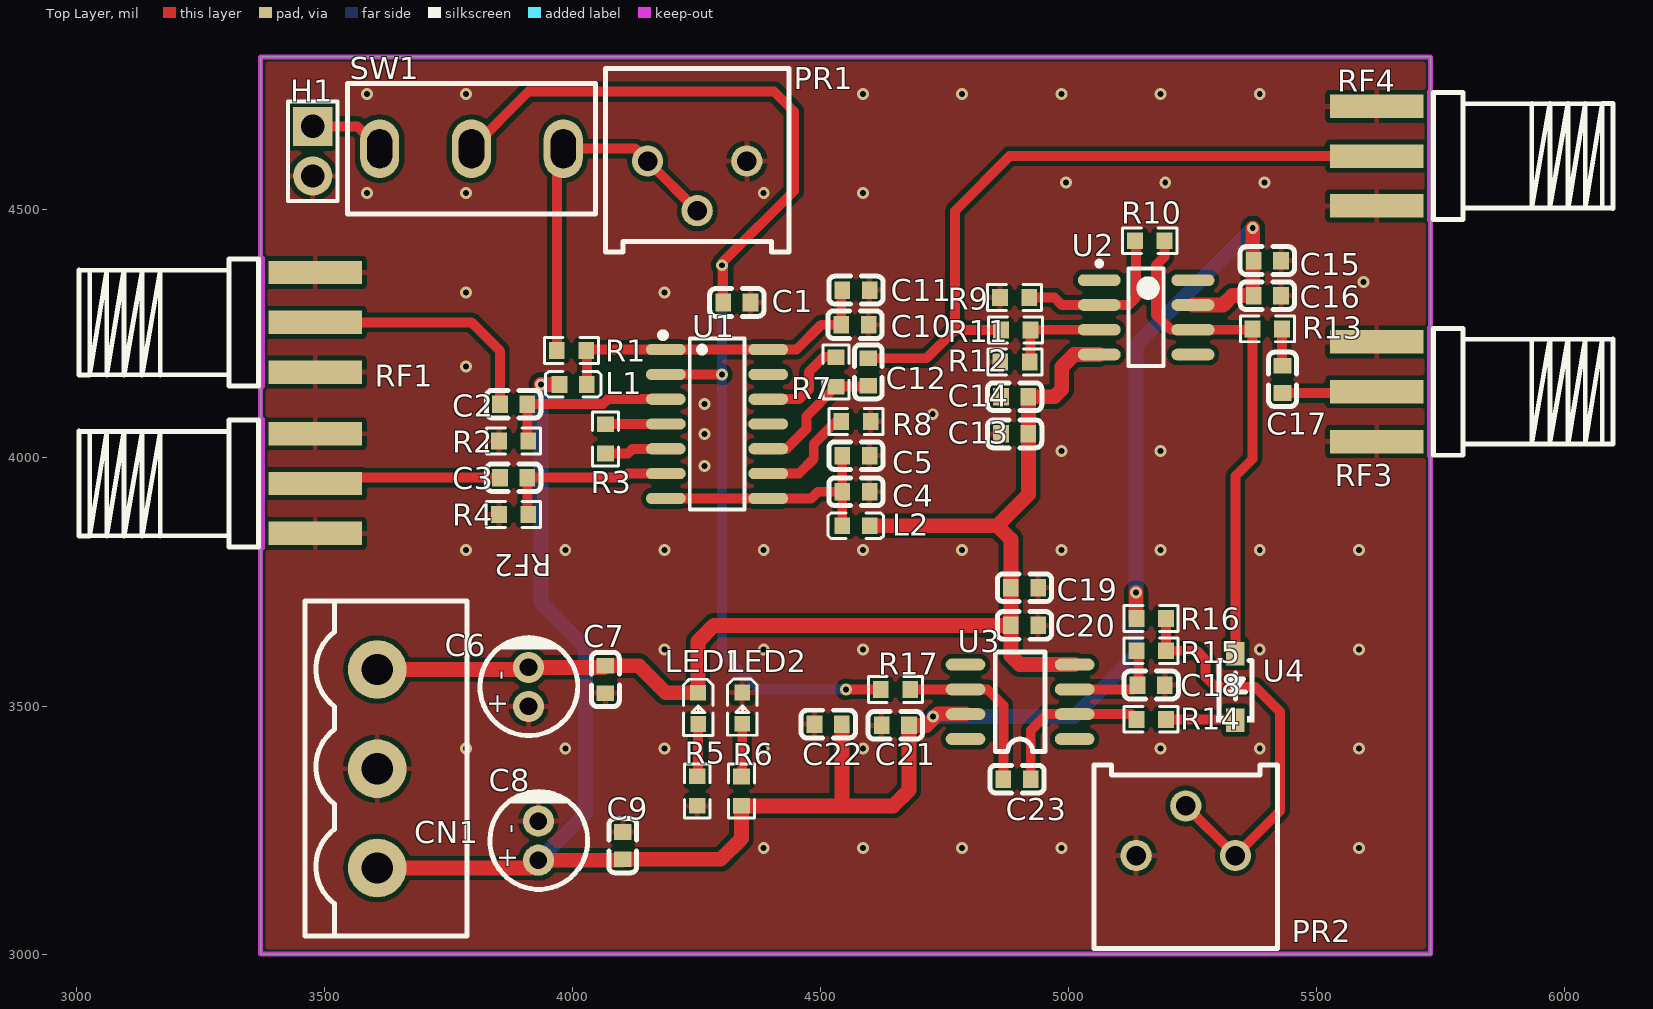
[diagram p0: Top Layer view]
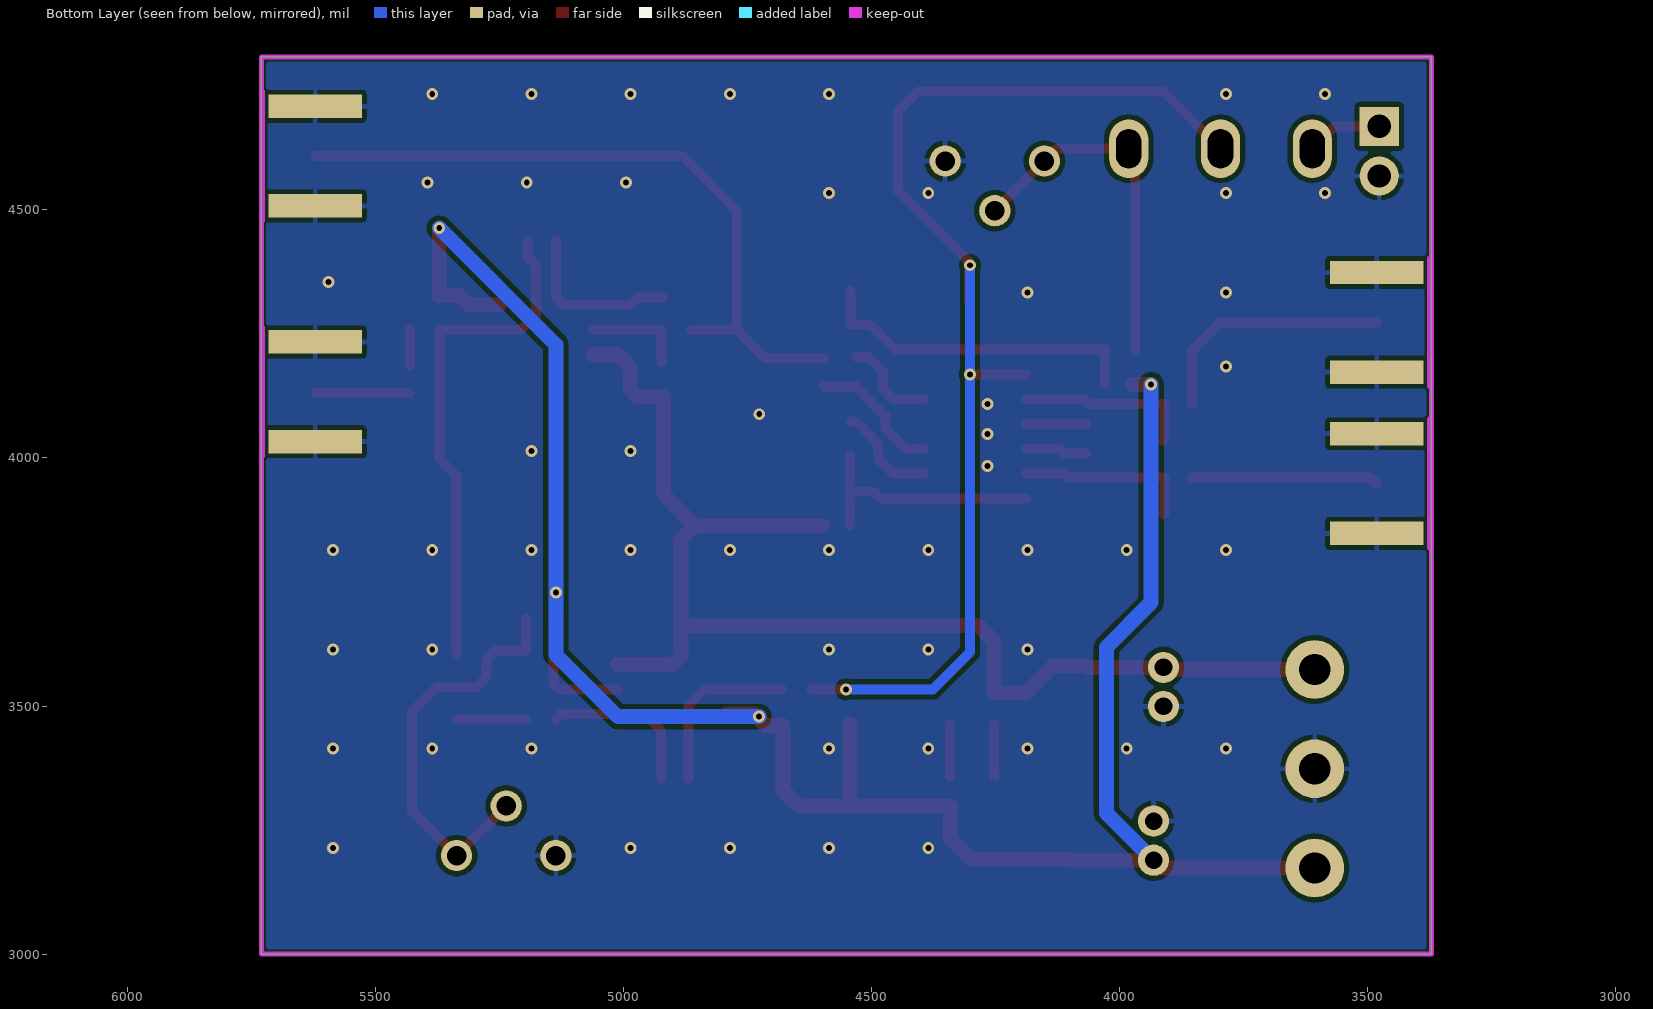
[diagram p1: Bottom Layer view, seen from below]
# Altium PCB MISC52012.pcbdoc
Units mil, origin at the board's own origin, x right, y up, seen from the top; angles counter-clockwise.
Board outline 2358.5 x 1808.5 mil, 2 copper layers (Top Layer, Bottom Layer), stack 62.206 mil thick; 57 components, 30 nets, 154 pads, 59 vias.

## Layer stack, top to bottom
Top Solder Mask Layer: solder mask 0.394, Dk 3.3
Top Layer: signal copper 1.379
Dielectric 1: surface 59.449, FR4, Dk 4.5
Bottom Layer: signal copper 1.378
Bottom Solder Mask Layer: solder mask 0.394, Dk 3.3

## Board outline
3371.1,4808.5 3371.1,3000 5729.61,3000 5729.61,4808.5

## Design rules (kind name [scope] priority, off if disabled: settings)
BoardOutlineClearance copperThickness2oz_1 [All] p2 off: genericclearance=7.99 ignorepadtopadclearanceinfootprint=FALSE except(0: Arc-SplitContinuation Track-SplitContinuation SMDPad-SplitContinuation THPad-SplitContinuation Via-SplitContinuation Fill-SplitContinuation Region-SplitContinuation Poly-SplitContinuation Text-SplitContinuation Hole-SplitContinuation; 5.98: Arc-CutoutEdge Track-CutoutEdge SMDPad-CutoutEdge THPad-CutoutEdge Via-CutoutEdge Text-CutoutEdge; 6.9: Hole-OutlineEdge Hole-CutoutEdge; 10: Poly-OutlineEdge Poly-CutoutEdge; 11.81: Arc-OutlineEdge Track-OutlineEdge SMDPad-OutlineEdge THPad-OutlineEdge Via-OutlineEdge Fill-OutlineEdge Region-OutlineEdge Text-OutlineEdge Fill-CutoutEdge Region-CutoutEdge)
BoardOutlineClearance Plane_innerPlane_1 [All] p4 off: genericclearance=4.02 ignorepadtopadclearanceinfootprint=FALSE except(0: Arc-SplitContinuation Track-SplitContinuation SMDPad-SplitContinuation THPad-SplitContinuation Via-SplitContinuation Fill-SplitContinuation Region-SplitContinuation Poly-SplitContinuation Text-SplitContinuation Hole-SplitContinuation; 5.98: Arc-CutoutEdge Track-CutoutEdge SMDPad-CutoutEdge THPad-CutoutEdge Via-CutoutEdge Text-CutoutEdge; 6.9: Hole-OutlineEdge Hole-CutoutEdge; 10: Poly-OutlineEdge Poly-CutoutEdge; 11.81: Arc-OutlineEdge Track-OutlineEdge SMDPad-OutlineEdge THPad-OutlineEdge Via-OutlineEdge Fill-OutlineEdge Region-OutlineEdge Text-OutlineEdge Fill-CutoutEdge Region-CutoutEdge)
BoardOutlineClearance Copper_copperRegion_1 [All] p6 off: genericclearance=4.02 ignorepadtopadclearanceinfootprint=FALSE except(0: Arc-SplitContinuation Track-SplitContinuation SMDPad-SplitContinuation THPad-SplitContinuation Via-SplitContinuation Fill-SplitContinuation Region-SplitContinuation Poly-SplitContinuation Text-SplitContinuation Hole-SplitContinuation; 5.98: Arc-CutoutEdge Track-CutoutEdge SMDPad-CutoutEdge THPad-CutoutEdge Via-CutoutEdge Text-CutoutEdge; 6.9: Hole-OutlineEdge Hole-CutoutEdge; 10: Poly-OutlineEdge Poly-CutoutEdge; 11.81: Arc-OutlineEdge Track-OutlineEdge SMDPad-OutlineEdge THPad-OutlineEdge Via-OutlineEdge Fill-OutlineEdge Region-OutlineEdge Text-OutlineEdge Fill-CutoutEdge Region-CutoutEdge)
BoardOutlineClearance copperThickness1oz_1 [All] p8: genericclearance=4.02 ignorepadtopadclearanceinfootprint=FALSE except(0: Arc-SplitContinuation Track-SplitContinuation SMDPad-SplitContinuation THPad-SplitContinuation Via-SplitContinuation Fill-SplitContinuation Region-SplitContinuation Poly-SplitContinuation Text-SplitContinuation Hole-SplitContinuation; 5.98: Arc-CutoutEdge Track-CutoutEdge SMDPad-CutoutEdge THPad-CutoutEdge Via-CutoutEdge Text-CutoutEdge; 6.9: Hole-OutlineEdge Hole-CutoutEdge; 10: Poly-OutlineEdge Poly-CutoutEdge; 11.81: Arc-OutlineEdge Track-OutlineEdge SMDPad-OutlineEdge THPad-OutlineEdge Via-OutlineEdge Fill-OutlineEdge Region-OutlineEdge Text-OutlineEdge Fill-CutoutEdge Region-CutoutEdge)
Clearance copperThickness2oz [All] p1 off: gap=7.99 ignorepadtopadclearanceinfootprint=FALSE except(5.98: SMDPad-Track SMDPad-SMDPad THPad-Track SMDPad-THPad THPad-THPad Track-Via SMDPad-Via THPad-Via Via-Via Fill-SMDPad Region-SMDPad Fill-THPad Region-THPad Fill-Via Region-Via Fill-Fill Fill-Region Region-Region Arc-Track Arc-SMDPad Arc-THPad Arc-Via Fill-Arc Region-Arc Arc-Arc Text-Track SMDPad-Text Text-THPad Text-Via Fill-Text Region-Text Arc-Text Text-Text; 6.9: Hole-Track Hole-SMDPad Hole-THPad Hole-Via Fill-Hole Region-Hole Hole-Arc Hole-Text; 10: Poly-Track Poly-SMDPad Poly-THPad Poly-Via Poly-Fill Poly-Region Poly-Poly Poly-Arc Poly-Text Poly-Hole; 11.81: Fill-Track Region-Track)
Clearance Plane_innerPlane [All] p3 off: gap=4.02 ignorepadtopadclearanceinfootprint=FALSE except(5.98: SMDPad-Track SMDPad-SMDPad THPad-Track SMDPad-THPad THPad-THPad Track-Via SMDPad-Via THPad-Via Via-Via Fill-SMDPad Region-SMDPad Fill-THPad Region-THPad Fill-Via Region-Via Fill-Fill Fill-Region Region-Region Arc-Track Arc-SMDPad Arc-THPad Arc-Via Fill-Arc Region-Arc Arc-Arc Text-Track SMDPad-Text Text-THPad Text-Via Fill-Text Region-Text Arc-Text Text-Text; 6.9: Hole-Track Hole-SMDPad Hole-THPad Hole-Via Fill-Hole Region-Hole Hole-Arc Hole-Text; 10: Poly-Track Poly-SMDPad Poly-THPad Poly-Via Poly-Fill Poly-Region Poly-Poly Poly-Arc Poly-Text Poly-Hole; 11.81: Fill-Track Region-Track)
Clearance Copper_copperRegion [All] p5 off: gap=4.02 ignorepadtopadclearanceinfootprint=FALSE except(5.98: SMDPad-Track SMDPad-SMDPad THPad-Track SMDPad-THPad THPad-THPad Track-Via SMDPad-Via THPad-Via Via-Via Fill-SMDPad Region-SMDPad Fill-THPad Region-THPad Fill-Via Region-Via Fill-Fill Fill-Region Region-Region Arc-Track Arc-SMDPad Arc-THPad Arc-Via Fill-Arc Region-Arc Arc-Arc Text-Track SMDPad-Text Text-THPad Text-Via Fill-Text Region-Text Arc-Text Text-Text; 6.9: Hole-Track Hole-SMDPad Hole-THPad Hole-Via Fill-Hole Region-Hole Hole-Arc Hole-Text; 10: Poly-Track Poly-SMDPad Poly-THPad Poly-Via Poly-Fill Poly-Region Poly-Poly Poly-Arc Poly-Text Poly-Hole; 11.81: Fill-Track Region-Track)
Clearance copperThickness1oz [All] p7: gap=4.02 ignorepadtopadclearanceinfootprint=FALSE except(5.98: SMDPad-Track SMDPad-SMDPad THPad-Track SMDPad-THPad THPad-THPad Track-Via SMDPad-Via THPad-Via Via-Via Fill-SMDPad Region-SMDPad Fill-THPad Region-THPad Fill-Via Region-Via Fill-Fill Fill-Region Region-Region Arc-Track Arc-SMDPad Arc-THPad Arc-Via Fill-Arc Region-Arc Arc-Arc Text-Track SMDPad-Text Text-THPad Text-Via Fill-Text Region-Text Arc-Text Text-Text; 6.9: Hole-Track Hole-SMDPad Hole-THPad Hole-Via Fill-Hole Region-Hole Hole-Arc Hole-Text; 10: Poly-Track Poly-SMDPad Poly-THPad Poly-Via Poly-Fill Poly-Region Poly-Poly Poly-Arc Poly-Text Poly-Hole; 11.81: Fill-Track Region-Track)
DiffPairsRouting differentialPair [All] p1: maxlimit=6 minlimit=6 mostfreqgap=6 toplayer_minwidth=5 toplayer_prefwidth=10 toplayer_maxwidth=100 toplayer_mingap=6 toplayer_prefgap=6 toplayer_maxgap=6 bottomlayer_minwidth=5 bottomlayer_prefwidth=10 bottomlayer_maxwidth=100 bottomlayer_mingap=6 bottomlayer_prefgap=6 bottomlayer_maxgap=6 maxuncoupledlength=10
HoleToHoleClearance otherClearance [All] p1: gap=11.81 allowstackedmicrovias=TRUE
Length netLength [All] p1: minlimit=0 maxlimit=0
PasteMaskExpansion pasteMaskExpansion [All] p1: expansion=0
PlaneConnect innerPlane [All] p1: planeconnectstyle=Relief reliefexpansion=20 reliefentries=4 reliefconductorwidth=10 reliefairgap=10
PolygonConnect copperRegion [All] p1: connectstyle=Relief reliefconductorwidth=10 reliefentries=4 polygonreliefangle="90 Angle" airgapwidth=10 via.connectstyle=Relief via.reliefconductorwidth=10 via.reliefentries=4 via.polygonreliefangle="90 Angle" via.airgapwidth=10
RoutingVias viaSize [All] p1: holewidth=12.01 width=24.02 viastyle="Through Hole" minholewidth=11.81 minwidth=19.68 maxholewidth=248.03 maxwidth=393.7
SolderMaskExpansion solderMaskExpansion [IsVia] p1: expansion=-1000 istentingtop=TRUE
SolderMaskExpansion solderMaskExpansion [All] p2: expansion=2 istentingtop=FALSE
Width copperThickness2oz_2 [All] p1 off: maxlimit=100 minlimit=8 preferedwidth=10
Width copperThickness1oz_2 [All] p2: maxlimit=100 minlimit=5 preferedwidth=10

## Components (designator, comment, footprint, x,y, rotation, side; value= is the part's Value field where it differs from the comment)
C1 "100nF" C0603 4331.1,4313.5 r180 top
C2 "100nF" C0603 3881.1,4108.5 r0 top
C3 "100nF" C0603 3881.1,3960.24 r0 top
C4 "100nF" C0603 4571.1,3931.94 r0 top
C5 "1uF" C0603 4571.1,4004.7 r180 top
C6 "10uF" CAP-TH_BD5.0-P2.00-D0.5-FD-A 3911.1,3538.5 r90 top
C7 "100nF" C0603 4066.1,3553.5 r90 top
C8 "10uF" CAP-TH_BD5.0-P2.00-D0.5-FD-A 3931.1,3228.5 r90 top
C9 "100nF" C0603 4101.1,3218.5 r270 top
C10 "1uF" C0603 4569.1,4268.56 r0 top
C11 "100nF" C0603 4571.1,4338.5 r0 top
C12 "100nF" C0603 4596.1,4173.5 r90 top
C13 "100nF" C0603 4891.1,4048.5 r0 top
C14 "1uF" C0603 4891.1,4123.5 r0 top
C15 "1uF" C0603 5400.45,4397.98 r0 top
C16 "100nF" C0603 5400.45,4327.19 r0 top
C17 "100nF" C0603 5431.1,4158.5 r270 top
C18 "100nF" C0603 5166.33,3542.25 r180 top
C19 "100nF" C0603 4910.99,3738.51 r180 top
C20 "1uF" C0603 4911,3662.53 r180 top
C21 "100nF" C0603 4650.47,3461.07 r180 top
C22 "1uF" C0603 4515.28,3463.51 r180 top
C23 "100nF" C0603 4896,3352.53 r180 top
CN1 "WJ2EDGVC-5.08-03P-14-00A" CONN-TH_3P-P5.08-WJ2EDGVC-3P 3606.1,3373.5 r270 top
H1 "PZ254V-11-02P" HDR-TH_2P-P2.54-V-M 3476.1,4618.5 r270 top
L1 "10uH" L0603 4001.1,4148.5 r0 top
L2 "10uH" L0603 4571.1,3863.5 r180 top
LED1 "" LED_0603 4253.2,3493.3 r270 top
LED2 "" LED_0603 4342.17,3493.79 r270 top
PR1 "10K" R_3386P 4251.1,4598.5 r90 top
PR2 "10K" R_3386P 5236.1,3198.5 r270 top
R1 "10K" R0603 3997.75,4216.58 r180 top
R2 "51R" R0603 3881.11,4034.38 r180 top
R3 "10" R0603 4066.1,4038.5 r90 top
R4 "50R" R0603 3881.11,3886.12 r0 top
R5 "1K" R0603 4251.1,3328.5 r90 top
R6 "1K" R0603 4340.27,3328.37 r90 top
R7 "1K" R0603 4531.1,4173.5 r270 top
R8 "0" R0603 4571.1,4073.5 r180 top
R9 "51R" R0603 4891.1,4323.5 r0 top
R10 "1K" R0603 5163.52,4437.98 r0 top
R11 "10R" R0603 4893.16,4257.98 r0 top
R12 "51R" R0603 4891.78,4193.5 r0 top
R13 "10R" R0603 5400.46,4260.34 r0 top
R14 "1K" R0603 5166.33,3473.17 r0 top
R15 "100" R0603 5166.33,3611.33 r0 top
R16 "3K" R0603 5166.33,3676.47 r180 top
R17 "100" R0603 4650.74,3533.17 r0 top
RF1 "6GHz" SMA-SMD_BWSMA-KE-P001 3481.1,4273.5 r180 top
RF2 "6GHz" SMA-SMD_BWSMA-KE-P001 3481.1,3948.5 r180 top
RF3 "6GHz" SMA-SMD_BWSMA-KE-P001 5621.1,4133.5 r0 top
RF4 "6GHz" SMA-SMD_BWSMA-KE-P001 5621.1,4608.5 r0 top
SW1 "SS-12D10L5" SW-TH_SS-12D10L5 3796.1,4623.5 r180 top
U1 "VCA821ID" SOIC-14_L8.7-W3.9-P1.27-LS6.0-BL 4291.1,4068.5 r270 top
U2 "OPA695" SOIC-8 5156.1,4283.5 r0 top
U3 "OPA820" SOP8 5011,3432.53 r180 top
U4 "1N4150" SOD-123_L2.7-W1.6-LS3.7-RD-1 5336.1,3538.5 r90 top

## Footprints (in the part's own frame and the unit in brackets; to place one, negate y for a bottom-side part, rotate by r counter-clockwise, add the part's x,y. Pads: shape width x height; smd on the part's side, far side on the other; paste and mask are expansions set on the pad)
C0603 [mm]
  rect 0.8x0.9 smd: 1(-0.7,0) 2(0.7,0)
  silkscreen extent -1.39,-0.71 1.39,0.71
CAP-TH_BD5.0-P2.00-D0.5-FD-A [mm]
  round 1.6 hole 0.9 paste+0 mask+0.05: 1(-1,0) 2(1,0)
  silkscreen extent -2.49,-2.52 2.6,2.49
CONN-TH_3P-P5.08-WJ2EDGVC-3P [mm]
  round 3 hole 1.6 paste+0 mask+0.05: 1(-5.08,0) 2(0,0) 3(5.08,0)
  silkscreen extent -8.58,-3.7 8.57,4.6
HDR-TH_2P-P2.54-V-M [mm]
  rect 2x2 hole 1.2: 1(-1.27,0)
  round 2 hole 1.2: 2(1.27,0)
  silkscreen extent -2.54,-1.27 2.54,1.27
L0603 [mm]
  rect 0.8x0.864 smd paste-100 mask+0.051: 1(-0.7,0) 2(0.7,0)
  silkscreen extent -1.42,-0.65 1.42,0.65
LED_0603 [mil]
  rect 31.5x31.5 smd paste+0 mask+2: 1(-33.5,-0.4) 2(29.5,-0.2)
  silkscreen extent -61,-30 53,30
R0603 [mil]
  rect 31.75x34.02 smd paste-3937.01 mask+2: 1(-29.66,0) 2(29.66,0)
  silkscreen extent -55,-26 55,26
R_3386P [mil]
  round 63 hole 39.4 paste+0 mask+2: 1(0,-100) 2(-100,0) 3(0,100)
  silkscreen extent -183,-185 187,185
SMA-SMD_BWSMA-KE-P001 [mm]
  rect 4.8x1.2 smd: 1(0,-2.55) 2(0,2.55) 5(0,0)
  rect 4.8x1.2 smd far side: 3(0,2.55) 4(0,-2.55)
  Board Outline Layer lines w0.254: 2.7,3.3 2.7,-3.3
  silkscreen extent 2.89,-3.25 12.1,3.25
SOD-123_L2.7-W1.6-LS3.7-RD-1 [mm]
  rect 1.2x0.95 smd: 1(-1.7,0) 2(1.7,0)
  silkscreen extent -1.81,-0.98 1.35,0.98
SOIC-8 [mm]
  oval 2.2x0.6 smd: 1(-2.4,1.905) 2(-2.4,0.635) 3(-2.4,-0.635) 4(-2.4,-1.905) 5(2.4,-1.905) 6(2.4,-0.635) 7(2.4,0.635) 8(2.4,1.905)
  silkscreen extent -2.52,-2.5 0.9,2.88
SOIC-14_L8.7-W3.9-P1.27-LS6.0-BL [mil]
  oval 22.6x80.24 smd: 1(-150,-103.11) 2(-100,-103.11) 3(-50,-103.11) 4(0,-103.11) 5(50,-103.11) 6(100,-103.11) 7(150,-103.11) 8(150,103.11) 9(100,103.11) 10(50,103.11) 11(0,103.11) 12(-50,103.11) 13(-100,103.11) 14(-150,103.11)
  silkscreen extent -185,-115 172,55
SOP8 [mil]
  oval 80x24 smd: 1(-1,-1) 2(-1,-51) 3(-1,-101) 4(-1,-151) 5(219,-151) 6(219,-101) 7(219,-51) 8(219,-1)
  silkscreen extent 59,-176 159,24
SW-TH_SS-12D10L5 [mm]
  oval 2x3 hole 1.3 slot 2 at 90 deg: 1(-4.7,0) 2(0,0) 3(4.7,0)
  silkscreen extent -6.35,-3.35 6.35,3.35

## Via types
v1: diameter 24.02, hole 12, Top Layer to Bottom Layer, 59 vias

## Nets (pads, with @x,y where several pads share a name; then routed paths per layer and width w, separated by ;. In a path a pad name is that pad's centre, name@x,y a point inside that pad or via, vN(x,y) a via of type N, cw(c..) or ccw(c..) an arc to the next point about the centre after c; other vN are vias at no path point)
5V: C8.1 C9.2 C15.1 C16.1 C21.1 C22.1 CN1.3 L1.1 R6.1 R16.2 U2.7 U3.7 | length 4406.3
  Top Layer w30: CN1.3 3915.48,3173.5 C8.1 4099.29,3189.13 C9.2 4298.54,3190.94 4340.27,3232.67 R6.1 4542.7,3298.71 ; v1(3936.1,4148.5) L1.1 ; C22.1 4542.84,3298.84 4542.7,3298.71 ; U3.7 4736.13,3483.53 4713.67,3461.07 C21.1 4678.03,3330.43 4646.31,3298.71 4542.7,3298.71 ; v1(5136.1,3728.5) 5136.1,3677.03 R16.2 ; U2.7 5311.1,4308.5 5329.78,4327.19 C16.1 5371.1,4328.98 v1(5371.1,4463.5)
  Bottom Layer w30: C8.1 4026.1,3284.13 4026.1,3618.5 3936.1,3708.5 v1(3936.1,4148.5) ; v1(4726.1,3478.5) 5011.1,3478.5 5136.1,3603.5 v1(5136.1,3728.5) 5136.1,4228.5 v1(5371.1,4463.5)
$1N219: C10.1 C11.1 L1.2 R1.1 U1.1 U1.14 | length 675
  Top Layer w20: L1.2 4028.66,4215.33 R1.1 4029.33,4218.5 U1.1 U1.14 4451.1,4218.5 4501.16,4268.56 C10.1 4541.54,4336.5 C11.1
$1N498: PR1.2 PR1.3 R1.2 SW1.1 | length 734.1
  Top Layer w20: R1.2 3968.09,4610.45 SW1.1 4126.1,4623.5 PR1.3 PR1.2
$1N910: H1.1 SW1.3 | length 153.6
  Top Layer w20: H1.1 3566.06,4668.5 SW1.3
$1N1030: C2.2 R2.1 U1.3 | length 358.5
  Top Layer w20: R2.1 3908.66,4036.48 C2.2 4061.1,4108.5 4071.1,4118.5 U1.3
$1N1197: C2.1 RF1.5 | length 503.8
  Top Layer w20: RF1.5 3796.11,4273.5 3853.54,4216.06 C2.1
$1N1319: R3.2 U1.4 | length 122
  Top Layer w20: R3.2 4066.44,4068.5 U1.4
$1N1323: R3.1 U1.5 | length 125.9
  Top Layer w20: R3.1 4111.44,4008.84 4121.1,4018.5 U1.5
$1N1332: C3.2 R4.2 U1.6 | length 357.7
  Top Layer w20: R4.2 3908.66,3888.22 C3.2 4102.84,3960.24 4111.1,3968.5 U1.6
$1N1471: C3.1 RF2.5 | length 377.3
  Top Layer w20: RF2.5 3492.84,3960.24 C3.1
$1N1598: C4.1 C5.2 L2.2 U1.7 U1.8 | length 502.3
  Top Layer w20: U1.7 U1.8 4481.1,3918.5 4494.54,3931.94 C4.1 ; L2.2 C4.1 ; C5.2 C4.1
$1N2316: LED1.2 R5.2 | length 106.4
  Top Layer w20: R5.2 4253,3360.06 LED1.2
$1N2422: LED2.2 R6.2 | length 107
  Top Layer w20: R6.2 4341.97,3359.73 LED2.2
$1N2806: R7.1 U1.12 | length 192.5
  Top Layer w20: U1.12 4456.1,4118.5 4476.1,4138.5 4476.1,4173.5 4505.76,4203.16 R7.1
$1N2903: C12.1 R7.2 U1.10 | length 269.5
  Top Layer w20: U1.10 4431.1,4018.5 4471.1,4058.5 4471.1,4083.84 R7.2 4594,4143.84 C12.1
$1N2974: C12.2 R11.1 RF4.5 | length 1427.3
  Top Layer w20: C12.2 4713.66,4201.06 4770.57,4257.98 ; R11.1 4770.57,4257.98 ; RF4.5 4881.11,4608.51 4770.57,4497.98 4770.57,4257.98
$1N3011: R8.2 U1.9 | length 208.3
  Top Layer w20: U1.9 4456.1,3968.5 4486.1,3998.5 4486.1,4028.5 4531.1,4073.5 R8.2
$1N3387: R10.2 R13.1 U2.6 U4.2 | length 1033.7
  Top Layer w20: R10.2 5193.18,4405.58 5176.1,4388.5 5176.1,4288.5 5206.1,4258.5 U2.6 5368.95,4258.5 R13.1 5370.8,3998.2 5336.1,3963.5 U4.2
$1N3468: R11.2 R12.2 U2.3 | length 204.1
  Top Layer w20: R12.2 4922.82,4194.88 R11.2 4923.35,4258.5 U2.3
$1N3475: R9.2 R10.1 U2.2 | length 343.2
  Top Layer w20: R9.2 4971.1,4323.5 4986.1,4308.5 U2.2 5121.1,4308.5 5136.1,4323.5 5136.1,4435.73 R10.1
$1N4114: C17.1 R13.2 | length 74.7
  Top Layer w20: R13.2 5430.12,4187.05 C17.1
$1N4255: C23.1 R14.1 U3.2 | length 329.3
  Top Layer w20: C23.1 4923.56,3450.96 4956.13,3483.53 U3.2 5126.31,3483.53 R14.1
$1N4395: R14.2 U4.1 | length 140.8
  Top Layer w20: R14.2 5334.51,3473.17 U4.1
$1N4413: C18.2 R15.1 U3.3 | length 202.3
  Top Layer w20: U3.3 5130.05,3533.53 C18.2 5141.1,3544.58 5141.1,3606.9 R15.1
$1N4523: PR2.2 PR2.3 R15.2 R16.1 | length 835.3
  Top Layer w20: R16.1 R15.2 5258.28,3611.33 5276.1,3593.5 5276.1,3558.5 5296.1,3538.5 5376.1,3538.5 5426.1,3488.5 5426.1,3288.5 PR2.3 PR2.2
$1N5100: C23.2 R17.2 U3.6 | length 350.2
  Top Layer w20: R17.2 4791.63,3533.17 U3.6 4836.08,3533.53 4868.44,3501.17 C23.2
$1N5172: C17.2 RF3.5 | length 191.1
  Top Layer w20: C17.2 5618.54,4130.94 RF3.5
-5V: C6.2 C7.2 C13.2 C14.2 C19.2 C20.2 CN1.1 L2.1 LED1.1 U2.4 U3.4 | length 2577.1
  Top Layer w30: CN1.1 3906.74,3573.5 C6.2 4062.91,3577.87 C7.2 4133.54,3581.06 4187.8,3526.8 LED1.1 4252.8,3630.2 4285.13,3662.53 C20.2 ; L2.1 4856.1,3863.5 ; U3.4 4901.08,3583.53 4883.44,3601.17 C20.2 ; U2.4 5011.1,4208.5 4986.1,4183.5 4986.1,4138.5 4971.1,4123.5 C14.2 C13.2 4918.66,3926.06 4856.1,3863.5 ; 4856.1,3863.5 4883.43,3836.18 C19.2 C20.2
GND: C1.1 C4.2 C5.1 C6.1 C7.1 C8.2 C9.1 C10.2 C11.2 C13.1 C14.1 C15.2 C16.2 C18.1 C19.1 C20.1 C21.2 C22.2 CN1.2 H1.2 LED2.1 PR1.1 PR2.1 R2.2 R4.1 R5.1 R8.1 R9.1 R12.1 RF1.1 RF1.2 RF1.3 RF1.4 RF2.1 RF2.2 RF2.3 RF2.4 RF3.1 RF3.2 RF3.3 RF3.4 RF4.1 RF4.2 RF4.3 RF4.4 U1.11
  other v1: 4385.2,3214.1 4585.2,3214.1 4785.2,3214.1 4985.2,3214.1 5585.2,3214.1 3785.2,3414.1 3985.2,3414.1 4185.2,3414.1 4385.2,3414.1 4585.2,3414.1 5185.2,3414.1 5385.2,3414.1 5585.2,3414.1 4185.2,3614.1 4385.2,3614.1 4585.2,3614.1 5385.2,3614.1 5585.2,3614.1 3785.2,3814.1 3985.2,3814.1 4185.2,3814.1 4385.2,3814.1 4585.2,3814.1 4785.2,3814.1 4985.2,3814.1 5185.2,3814.1 5385.2,3814.1 5585.2,3814.1 4266.1,3983.82 4985.2,4014.1 5185.2,4014.1 4266.1,4048.5 4725.95,4088.22 4266.1,4108.5 3785.2,4184.34 3785.2,4333.92 4185.2,4333.92 5594.67,4355.04 3585.2,4533.92 3785.2,4533.92 4385.2,4533.92 4585.2,4533.92 4994.67,4555.04 5194.67,4555.04 5394.67,4555.04 3585.2,4733.92 3785.2,4733.92 4585.2,4733.92 4785.2,4733.92 4985.2,4733.92 5185.2,4733.92 5385.2,4733.92
VG: C1.2 R17.1 SW1.2 U1.2 | length 2402.5
  Top Layer w20: SW1.2 3911.1,4738.5 4406.1,4738.5 4446.1,4698.5 4446.1,4538.5 4303.54,4395.94 C1.2 ; U1.2 v1(4301.1,4168.5) ; v1(4551.1,3533.5) 4620.74,3533.5 R17.1
  Bottom Layer w20: v1(4301.1,4388.5) v1(4301.1,4168.5) 4301.1,3608.5 4376.1,3533.5 v1(4551.1,3533.5)
pads on no net: U1.13 U2.1 U2.5 U2.8 U3.1 U3.5 U3.8

## Polygon pours and split planes (outlines as drawn)
GND on Top Layer (solid, remove dead copper, pour order 0): 3371.1,4808.5 3371.1,3000 5729.61,3000 5729.61,4808.5
GND on Bottom Layer (solid, remove dead copper, pour order 2): 3371.1,4808.5 3371.1,3000 5729.61,3000 5729.61,4808.5

## Keep-outs
Board Outline Layer:
  the board outline again, w10